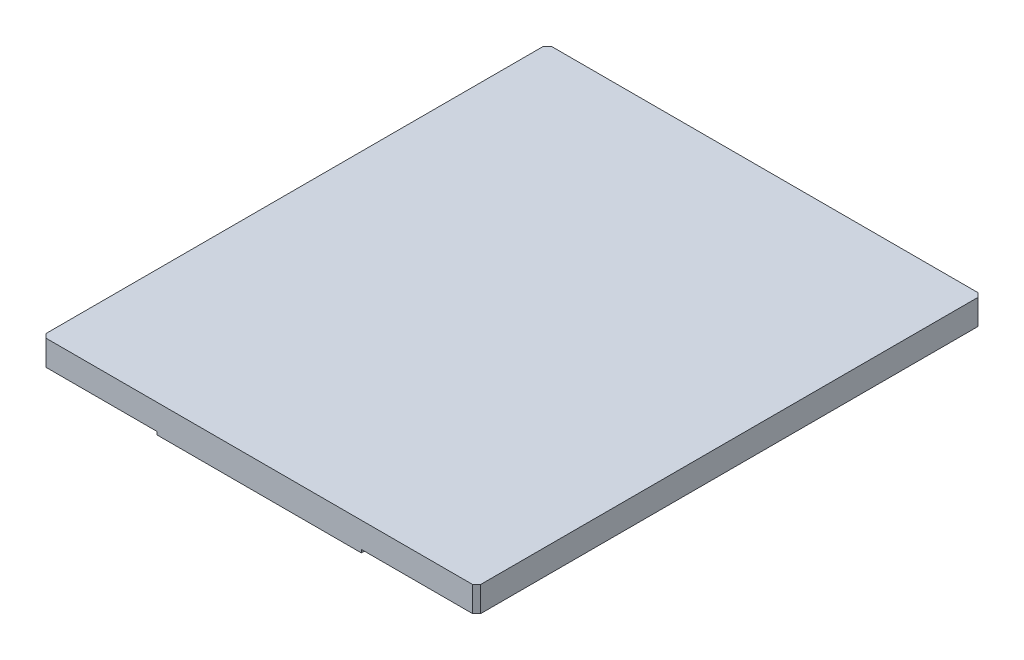
SolidWorks part; units mm, degrees
ref_plane "前视基准面" through (0, 0, 0) normal (0, 0, 1) x (1, 0, 0)
ref_plane "上视基准面" through (0, 0, 0) normal (0, 1, 0) x (1, 0, 0)
ref_plane "右视基准面" through (0, 0, 0) normal (1, 0, 0) x (0, 0, -1)
sketch "草图1" plane through (0, 0, 0) normal (0, 1, 0) x (1, 0, 0)
  line L1 (-107.5, -125) -> (107.5, -125)
  line L2 (-107.5, -125) -> (-107.5, 125)
  line L3 (-107.5, 125) -> (107.5, 125)
  line L4 (107.5, -125) -> (107.5, 125)
  line L5 (-107.5, -125) -> (107.5, 125) construction
  line L6 (-107.5, 125) -> (107.5, -125) construction
  point P0 (0, 0)
  dimension "D1" = 215
  dimension "D2" = 250
extrude "凸台-拉伸1" add sketch "草图1" along normal mid plane 14
sketch "草图2" plane through (0, -7, 0) normal (0, -1, 0) x (1, 0, 0)
  line L0 (-107.5, 125) -> (107.5, 125) construction
  line L1 (107.5, -125) -> (50.5, -125)
  line L2 (107.5, -125) -> (107.5, 125)
  line L3 (107.5, 125) -> (50.5, 125)
  line L4 (50.5, -125) -> (50.5, 125)
  line L6 (-107.5, -125) -> (-50.5, -125)
  line L7 (-107.5, -125) -> (-107.5, 125)
  line L8 (-107.5, 125) -> (-50.5, 125)
  line L9 (-50.5, -125) -> (-50.5, 125)
  dimension "D1" = 57
extrude "切除-拉伸1" cut sketch "草图2" against normal blind 1.5
sketch "草图3" plane through (0, 7, 0) normal (0, 1, 0) x (1, 0, 0)
  line L0 (-107.5, 125) -> (-107.5, -125) construction
  line L1 (42.5, -80) -> (-42.5, -80)
  line L2 (42.5, -80) -> (42.5, -32.5)
  line L3 (42.5, 80) -> (-42.5, 80)
  line L4 (-42.5, -80) -> (-42.5, -32.5)
  line L5 (42.5, -80) -> (-42.5, 80) construction
  line L6 (42.5, 80) -> (-42.5, -80) construction
  line L7 (-107.5, -125) -> (107.5, -125) construction
  line L8 (-42.5, -32.5) -> (42.5, -32.5)
  line L9 (-42.5, 32.5) -> (42.5, 32.5)
  line L10 (-42.5, 32.5) -> (-42.5, 80)
  line L11 (42.5, 32.5) -> (42.5, 80)
  point P0 (0, 0)
  dimension "D1" = 65
  dimension "D2" = 45
  dimension "D3" = 65
extrude "切除-拉伸2" [suppressed] cut sketch "草图3" against normal up to next
fillet "圆角1" [suppressed] radius 10
chamfer "倒角1" distance 2 angle 45 4 edges at (107.5, 0.75, -125) (-107.5, 0.75, -125) (-107.5, 0.75, 125) (107.5, 0.75, 125)
